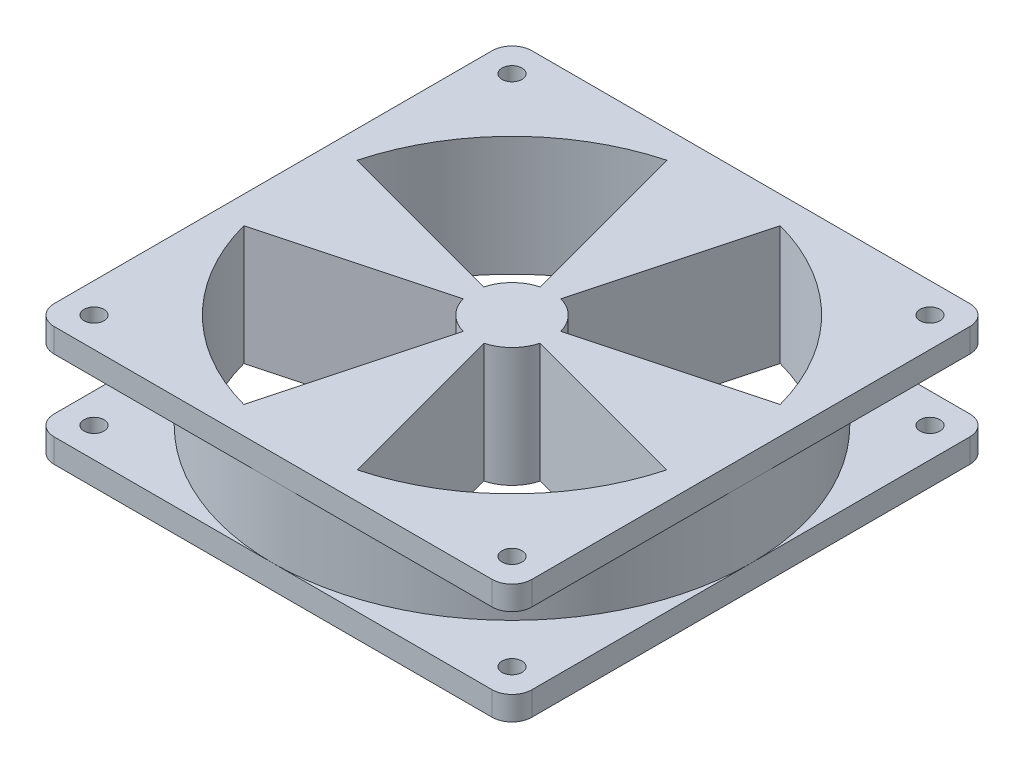
SolidWorks part; units mm, degrees
material "6061"
ref_plane "前视基准面" through (0, 0, 0) normal (0, 0, 1) x (1, 0, 0)
ref_plane "上视基准面" through (0, 0, 0) normal (0, 1, 0) x (1, 0, 0)
ref_plane "右视基准面" through (0, 0, 0) normal (1, 0, 0) x (0, 0, -1)
sketch "草图1" plane through (0, 0, 0) normal (0, 1, 0) x (1, 0, 0)
  line L1 (-60, 60) -> (60, 60)
  line L2 (-60, 60) -> (-60, -60)
  line L3 (-60, -60) -> (60, -60)
  line L4 (60, 60) -> (60, -60)
  line L5 (-60, 60) -> (60, -60) construction
  line L6 (-60, -60) -> (60, 60) construction
  point P0 (0, 0)
  dimension "D1" = 120
  dimension "D2" = 120
extrude "凸台-拉伸1" add sketch "草图1" along normal mid plane 30
sketch "草图3" plane through (0, 0, 0) normal (0, 1, 0) x (1, 0, 0)
  circle A0 centre (0, 0) radius 60
  circle A1 centre (0, 0) radius 90.7915
  dimension "D1" = 120
extrude "切除-拉伸1" cut sketch "草图3" against normal mid plane 18
sketch "草图4" plane through (0, 15, 0) normal (0, 1, 0) x (1, 0, 0)
  line L0 (0, 60) -> (0, -60) construction
  line L1 (60, 60) -> (-60, 60) construction
  line L2 (-60, -60) -> (60, -60) construction
  line L3 (-60, 0) -> (60, 0) construction
  line L4 (-60, 60) -> (-60, -60) construction
  line L5 (60, -60) -> (60, 60) construction
  circle A0 centre (-52.5, 52.5) radius 2.5
  circle A1 centre (-52.5, -52.5) radius 2.5
  circle A2 centre (52.5, -52.5) radius 2.5
  circle A3 centre (52.5, 52.5) radius 2.5
  dimension "D1" = 5
  dimension "D2" = 105
  dimension "D3" = 105
extrude "切除-拉伸3" cut sketch "草图4" against normal through all
fillet "圆角1" radius 5 8 edges at (-60, -12, 60) (-60, -12, -60) (60, -12, -60) (60, -12, 60) (-60, 12, 60) (-60, 12, -60) (60, 12, -60) (60, 12, 60)
sketch "草图5" plane through (0, 15, 0) normal (0, 1, 0) x (1, 0, 0)
  line L0 (0, 55) -> (0, -55) construction
  line L1 (-55, 0) -> (55, 0) construction
  line L2 (0, 0) -> (-14.235, 53.1259)
  line L3 (0, 0) -> (14.235, 53.1259)
  line L4 (0, 0) -> (-14.235, -53.1259)
  line L5 (0, 0) -> (14.235, -53.1259)
  line L6 (0, 0) -> (-53.1259, 14.235)
  line L7 (0, 0) -> (-53.1259, -14.235)
  line L8 (0, 0) -> (53.1259, -14.235)
  line L9 (0, 0) -> (53.1259, 14.235)
  circle A0 centre (0, 0) radius 10
  circle A1 centre (0, 0) radius 55
  dimension "D1" = 20
  dimension "D2" = 110
  dimension "D3" = 30
  dimension "D4" = 30
extrude "切除-拉伸4" cut sketch "草图5" against normal through all contours L2 A1 L6 A0 | L9 A1 L3 A0 | L5 A1 L8 A0 | L7 A1 L4 A0
